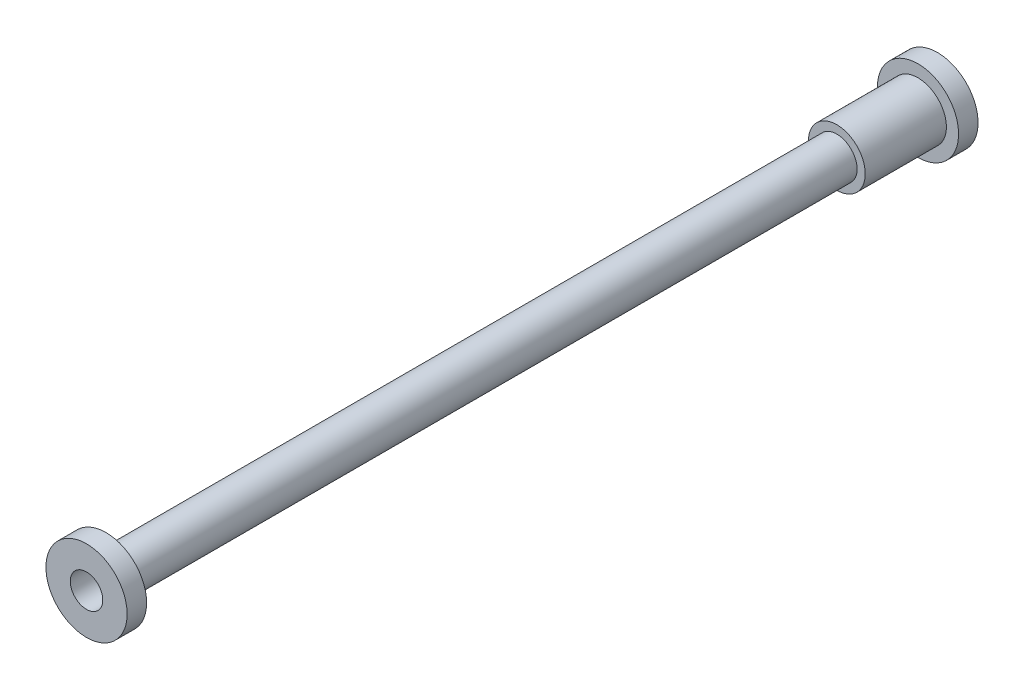
SolidWorks part; units mm, degrees
ref_plane "Front Plane" through (0, 0, 0) normal (0, 0, 1) x (1, 0, 0)
ref_plane "Top Plane" through (0, 0, 0) normal (0, 1, 0) x (1, 0, 0)
ref_plane "Right Plane" through (0, 0, 0) normal (1, 0, 0) x (0, 0, -1)
sketch "Sketch1" plane through (0, 0, 0) normal (0, 0, 1) x (1, 0, 0)
  circle A0 centre (0, 0) radius 12.5
  dimension "D1" = 25
extrude "Boss-Extrude1" add sketch "Sketch1" along normal blind 450
sketch "Sketch2" plane through (0, 0, 0) normal (0, 0, -1) x (-1, 0, 0)
  circle A0 centre (0, 0) radius 17.5
  dimension "D1" = 35
extrude "Boss-Extrude2" add sketch "Sketch2" along normal blind 50
sketch "Sketch3" plane through (0, 0, -50) normal (0, 0, -1) x (-1, 0, 0)
  circle A0 centre (0, 0) radius 25
  dimension "D1" = 50
extrude "Boss-Extrude3" add sketch "Sketch3" along normal blind 12
sketch "Sketch4" plane through (0, 0, 450) normal (0, 0, 1) x (1, 0, 0)
  circle A0 centre (0, 0) radius 25
  dimension "D1" = 50
extrude "Boss-Extrude4" add sketch "Sketch4" along normal blind 12
sketch "Sketch5" plane through (0, 0, 462) normal (0, 0, 1) x (1, 0, 0)
  circle A0 centre (0, 0) radius 10
  dimension "D1" = 20
extrude "Cut-Extrude1" cut sketch "Sketch5" against normal through all
